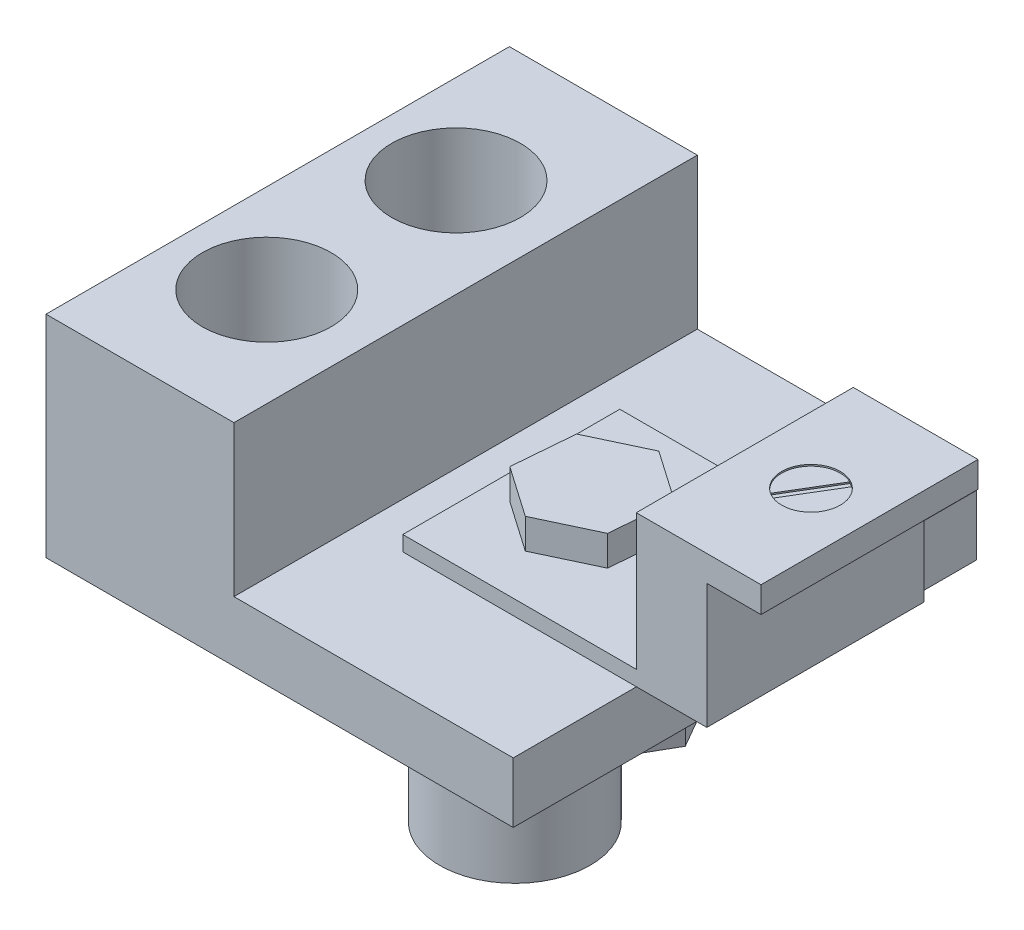
from build123d import *

# Parameters (mm, degrees)
BOSS_EXTRUDE1_DEPTH = 5
SKETCH2_R           = 5
BOSS_EXTRUDE2_DEPTH = 10
SKETCH3_W           = 31.008368254
SKETCH3_H           = 30.751916894
BOSS_EXTRUDE3_DEPTH = 4
SKETCH4_W           = 12.473016313
SKETCH4_H           = 30.751916894
BOSS_EXTRUDE4_DEPTH = 10
SKETCH5_W           = 20.18023145
SKETCH5_H           = 14.400921404
BOSS_EXTRUDE5_DEPTH = 1
BOSS_EXTRUDE6_DEPTH = 14.400921404
SKETCH7_R           = 4.270954595
CUT_EXTRUDE1_DEPTH  = 11
SKETCH8_R           = 1.943003429
CUT_EXTRUDE2_DEPTH  = 0.1
CUT_EXTRUDE3_DEPTH  = 0.1
BOSS_EXTRUDE7_DEPTH = 2


with BuildPart() as part:
    # Sketch1 → Boss-Extrude1 (new body)
    with BuildSketch(Plane(origin=(0, 0, 0), x_dir=(1, 0, 0), z_dir=(0, 1, 0))):
        Polygon((5.773502692, 10), (-5.773502692, 10), (-11.547005384, 0), (-5.773502692, -10), (5.773502692, -10), (11.547005384, 0), align=None)
    extrude(amount=BOSS_EXTRUDE1_DEPTH)

    # Sketch2 → Boss-Extrude2 (add)
    with BuildSketch(Plane.XZ):
        with Locations(Location((0.234789437, 0, 0), (0, 0, 270))):
            Circle(SKETCH2_R)
    extrude(amount=BOSS_EXTRUDE2_DEPTH)

    # Sketch3 → Boss-Extrude3 (add)
    with BuildSketch(Plane(origin=(0, 5, 0), x_dir=(1, 0, 0), z_dir=(0, 1, 0))):
        Rectangle(SKETCH3_W, SKETCH3_H)
    extrude(amount=BOSS_EXTRUDE3_DEPTH)

    # Sketch4 → Boss-Extrude4 (add)
    with BuildSketch(Plane(origin=(0, 9, 0), x_dir=(1, 0, 0), z_dir=(0, 1, 0))):
        with Locations((-9.267675971, 0)):
            Rectangle(SKETCH4_W, SKETCH4_H)
    extrude(amount=BOSS_EXTRUDE4_DEPTH)

    # Sketch5 → Boss-Extrude5 (add)
    with BuildSketch(Plane(origin=(0, 9, 0), x_dir=(1, 0, 0), z_dir=(0, 1, 0))):
        with Locations((10.090115725, 0)):
            Rectangle(SKETCH5_W, SKETCH5_H)
    extrude(amount=BOSS_EXTRUDE5_DEPTH)

    # Sketch6 → Boss-Extrude6 (add)
    with BuildSketch(Plane.XY.offset(7.200460702)):
        Polygon((20.18023145, 10), (20.18023145, 17.284010358), (23.772647306, 17.284010358), (23.772647306, 19), (15.494895542, 19), (15.494895542, 10), align=None)
    extrude(amount=-BOSS_EXTRUDE6_DEPTH)

    # Sketch7 → Cut-Extrude1 (cut)
    with BuildSketch(Plane(origin=(0, 19, 0), x_dir=(1, 0, 0), z_dir=(0, 1, 0))):
        with Locations(Location((-9.583665468, 5.917314438, 0), (0, 0, 270))):
            Circle(SKETCH7_R)
        with Locations(Location((-9.583665468, -6.64552011, 0), (0, 0, 270))):
            Circle(SKETCH7_R)
    extrude(amount=-CUT_EXTRUDE1_DEPTH, mode=Mode.SUBTRACT)

    # Sketch8 → Cut-Extrude2 (cut)
    with BuildSketch(Plane(origin=(0, 19, 0), x_dir=(1, 0, 0), z_dir=(0, 1, 0))):
        with Locations(Location((19.889507686, 0, 0), (0, 0, 270))):
            Circle(SKETCH8_R)
    extrude(amount=-CUT_EXTRUDE2_DEPTH, mode=Mode.SUBTRACT)

    # Sketch9 → Cut-Extrude3 (cut)
    with BuildSketch(Plane(origin=(0, 18.9, 0), x_dir=(1, 0, 0), z_dir=(0, 1, 0))):
        Polygon((18.714185293, -1.560675462), (20.714119659, 1.771187657), (21.064830078, 1.560675462), (19.064895713, -1.771187657), align=None)
    extrude(amount=-CUT_EXTRUDE3_DEPTH, mode=Mode.SUBTRACT)

    # Sketch10 → Boss-Extrude7 (add)
    with BuildSketch(Plane(origin=(0, 10, 0), x_dir=(1, 0, 0), z_dir=(0, 1, 0))):
        Polygon((5.703266191, 4.088977096), (1.990998258, 2.340859575), (1.648778474, -1.748117521), (5.018826623, -4.088977096), (8.731094556, -2.340859575), (9.07331434, 1.748117521), align=None)
    extrude(amount=BOSS_EXTRUDE7_DEPTH)


solid = part.part
